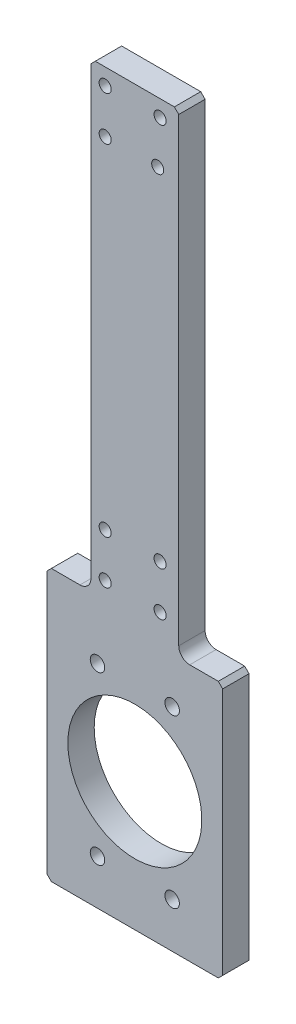
SolidWorks part; units mm, degrees
ref_plane "前视基准面" through (0, 0, 0) normal (0, 0, 1) x (1, 0, 0)
ref_plane "上视基准面" through (0, 0, 0) normal (0, 1, 0) x (1, 0, 0)
ref_plane "右视基准面" through (0, 0, 0) normal (1, 0, 0) x (0, 0, -1)
sketch "草图1" plane through (0, 0, 0) normal (0, 0, 1) x (1, 0, 0)
  line L1 (-40, -166.75) -> (40, -166.75)
  line L2 (-40, -166.75) -> (-40, 166.75)
  line L3 (-40, 166.75) -> (40, 166.75)
  line L4 (40, -166.75) -> (40, 166.75)
  line L5 (-40, -166.75) -> (40, 166.75) construction
  line L6 (-40, 166.75) -> (40, -166.75) construction
  point P0 (0, 0)
  dimension "D1" = 80
  dimension "D2" = 333.5
extrude "凸台-拉伸1" add sketch "草图1" along normal blind 12 contours L3 L4 L1 L2
chamfer "倒角1" distance 2 angle 45 4 edges at (-40, 166.75, 6) (40, 166.75, 6) (40, -166.75, 6) (-40, -166.75, 6)
sketch "草图9" plane through (0, 0, 0) normal (0, 0, -1) x (-1, 0, 0)
  line L0 (0, 0) -> (87.22, 0) construction
  point P18 (13.5, 139.25)
  point P19 (-11.5, 159.25)
  point P20 (-10.4189, 139.25)
  point P21 (13.5, 159.25)
  point P36 (-11.5, -15.75)
  point P39 (13.5, -15.75)
  point P42 (-11.5, -35.75)
  point P45 (13.5, -35.75)
hole_wizard "M5 六角圆柱头螺钉的柱形沉头孔1" positions "草图9" profile "草图8" counterbore size "M5" standard "GB" end condition through all
sketch "草图8" plane through (-13.5, -35.75, 0) normal (1, 0, 0) x (0, 1, 0)
  line L0 (0, 0) -> (0, 12)
  line L1 (0, 12) -> (2.75, 12)
  line L3 (2.75, 12) -> (2.75, 5.7)
  line L4 (2.75, 5.7) -> (5, 5.7)
  line L5 (5, 5.7) -> (5, 0)
  line L7 (5, 0) -> (0, 0)
  line L11 (0, -6.35) -> (0, 107.95) construction
  dimension "通孔孔直径" = 5.5
  dimension "通孔孔深度" = 12
  dimension "柱形沉头孔直径" = 10
  dimension "柱形沉头孔深度" = 5.7
sketch "草图10" plane through (0, 0, 12) normal (0, 0, 1) x (1, 0, 0)
  line L0 (-40, -164.75) -> (-40, 164.75) construction
  line L1 (-40, 166.75) -> (-20, 166.75)
  line L2 (-40, 166.75) -> (-40, -43.25)
  line L3 (-40, -43.25) -> (-20, -43.25)
  line L4 (-20, 166.75) -> (-20, -43.25)
  line L5 (-38, 166.75) -> (38, 166.75) construction
  line L6 (40, -164.75) -> (40, 164.75) construction
  line L8 (40, 166.75) -> (20, 166.75)
  line L9 (40, 166.75) -> (40, -49.75)
  line L10 (40, -49.75) -> (20, -49.75)
  line L11 (20, 166.75) -> (20, -49.75)
  dimension "D1" = 40
  dimension "D2" = 210
  dimension "D3" = 216.5
extrude "切除-拉伸1" cut sketch "草图10" against normal through all
chamfer "倒角2" distance 2 angle 45 4 edges at (-40, -43.25, 6) (40, -49.75, 6) (20, 166.75, 6) (-20, 166.75, 6)
fillet "圆角1" radius 5 2 edges at (-20, -43.25, 6) (20, -49.75, 6)
sketch "草图13" plane through (0, 0, 0) normal (0, 0, -1) x (-1, 0, 0)
  point P0 (-17, -70.25)
  point P3 (-17, -146.25)
  point P6 (17, -146.25)
  point P9 (17, -70.25)
hole_wizard "M6 六角圆柱头螺钉的柱形沉头孔1" positions "草图13" profile "草图12" counterbore size "M6" standard "GB" end condition through all
sketch "草图12" plane through (17, -70.25, 0) normal (1, 0, 0) x (0, 1, 0)
  line L0 (0, 0) -> (0, 12)
  line L1 (0, 12) -> (3.3, 12)
  line L3 (3.3, 12) -> (3.3, 6.8)
  line L4 (3.3, 6.8) -> (5.5, 6.8)
  line L5 (5.5, 6.8) -> (5.5, 0)
  line L7 (5.5, 0) -> (0, 0)
  line L11 (0, -6.35) -> (0, 107.95) construction
  dimension "通孔孔直径" = 6.6
  dimension "通孔孔深度" = 12
  dimension "柱形沉头孔直径" = 11
  dimension "柱形沉头孔深度" = 6.8
sketch "草图14" plane through (0, 0, 0) normal (0, 0, -1) x (-1, 0, 0)
  circle A0 centre (0, -108.25) radius 30.5
  dimension "D1" = 61
extrude "切除-拉伸2" cut sketch "草图14" against normal through all
